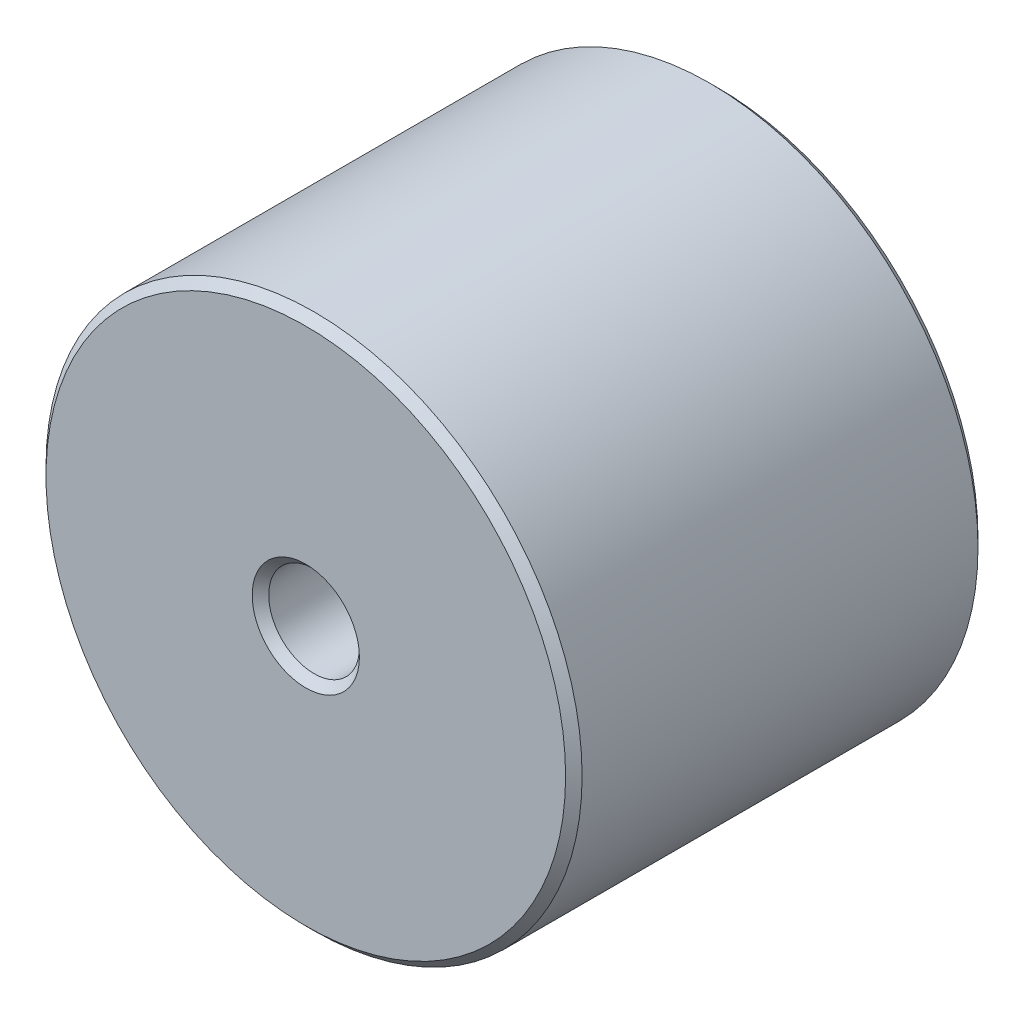
from build123d import *

# Parameters (mm, degrees)
SKETCH_1_R      = 32.5
SKETCH_1_R_2    = 5.5
EXTRUDE_1_DEPTH = 50
CHAMFER_1_SIZE  = 1


with BuildPart() as part:
    # 草图1 → 凸台-拉伸1 (new body)
    with BuildSketch(Plane.XY):
        Circle(SKETCH_1_R)
        Circle(SKETCH_1_R_2, mode=Mode.SUBTRACT)
    extrude(amount=EXTRUDE_1_DEPTH)

    # 倒角1
    chamfer_1_edges = [part.edges().sort_by_distance(p)[0] for p in [
        (-32.5, 0, 0),
        (-32.5, 0, 50),
        (-5.5, 0, 0),
        (-5.5, 0, 50),
    ]]
    chamfer(chamfer_1_edges, length=CHAMFER_1_SIZE)


solid = part.part
